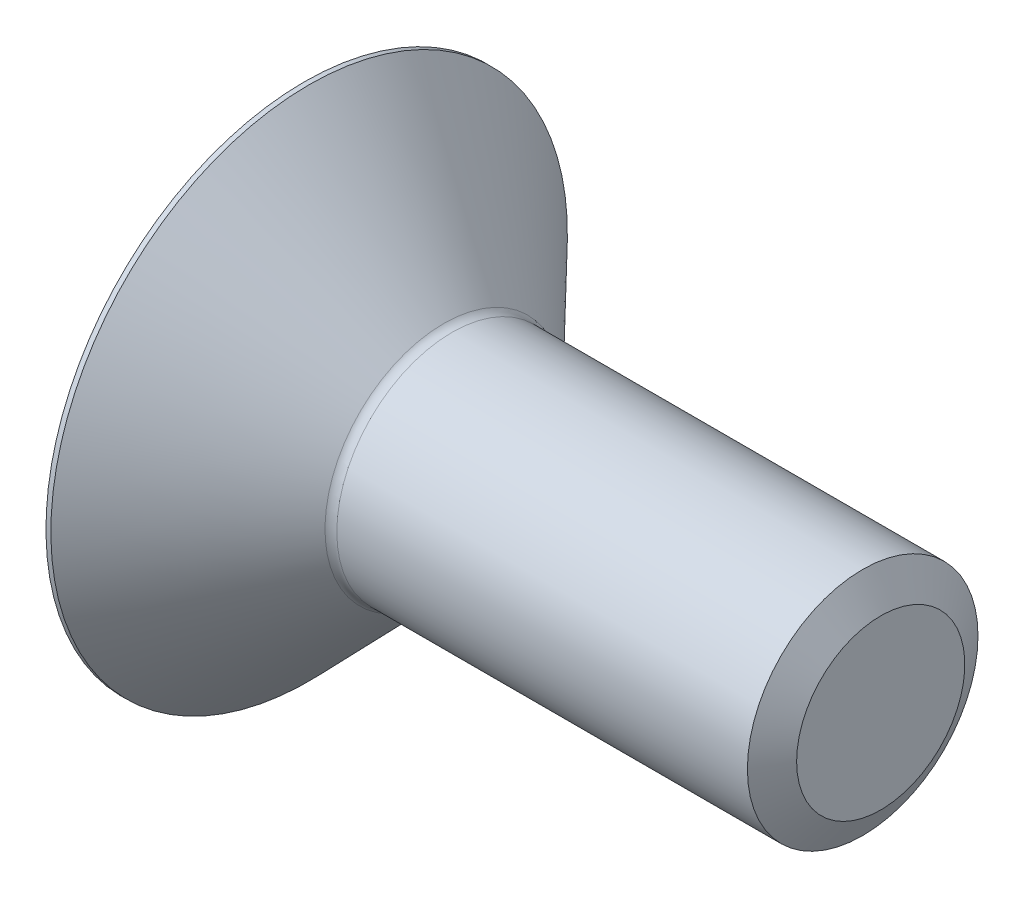
from build123d import *

# Parameters (mm, degrees)
CUT_EXTRUDE1_DEPTH = 5.06


with BuildPart() as part:
    # Sketch1 → Revolve1 (revolve)
    with BuildSketch(Plane.XY):
        with BuildLine():
            Line((0, 4), (-14.870210074, 4))
            ThreePointArc((-14.870210074, 4), (-15.026502525, 4.031798059), (-15.157945994, 4.122136652))
            Line((-15.157945994, 4.122136652), (-19.829816323, 8.96))
            Line((-19.829816323, 8.96), (-20, 8.96))
            Line((-20, 8.96), (-20, 0))
            Line((-20, 0), (0, 0))
            Line((0, 0), (0, 4))
        make_face()
    revolve(axis=Axis((0, 0, 0), (-1, 0, 0)))

    # Sketch2 → Cut-Extrude1 (cut)
    with BuildSketch(Plane.ZY.offset(20)):
        Polygon((0, 2.886751346), (-2.5, 1.443375673), (-2.5, -1.443375673), (0, -2.886751346), (2.5, -1.443375673), (2.5, 1.443375673), align=None)
    extrude(amount=-CUT_EXTRUDE1_DEPTH, mode=Mode.SUBTRACT)

    # Sketch6 → Revolve2 (revolve)
    with BuildSketch(Plane.XY, mode=Mode.PRIVATE) as revolve2_sk:
        Polygon((-17, 2.886751346), (-15.333333333, 0), (-14.22, 0), (-14.22, 2.886751346), align=None)
    revolve(revolve2_sk.sketch.rotate(Axis((-20, 0, 0), (1, 0, 0)), 90), axis=Axis((-20, 0, 0), (1, 0, 0)))

    # Sketch7 → Cut-Revolve2 (revolve, cut)
    with BuildSketch(Plane.XY):
        Polygon((-20, 2.886751346), (-20, 0), (-19.208, 0), align=None)
    revolve(axis=Axis((-20, 0, 0), (1, 0, 0)), mode=Mode.SUBTRACT)

    # Sketch4 → Cut-Revolve1 (revolve, cut)
    with BuildSketch(Plane.XY):
        Polygon((-0.625, 4), (0, 2.917468245), (0.625, 4), align=None)
    revolve(axis=Axis((-0.625, 0, 0), (1, 0, 0)), mode=Mode.SUBTRACT)


solid = part.part
